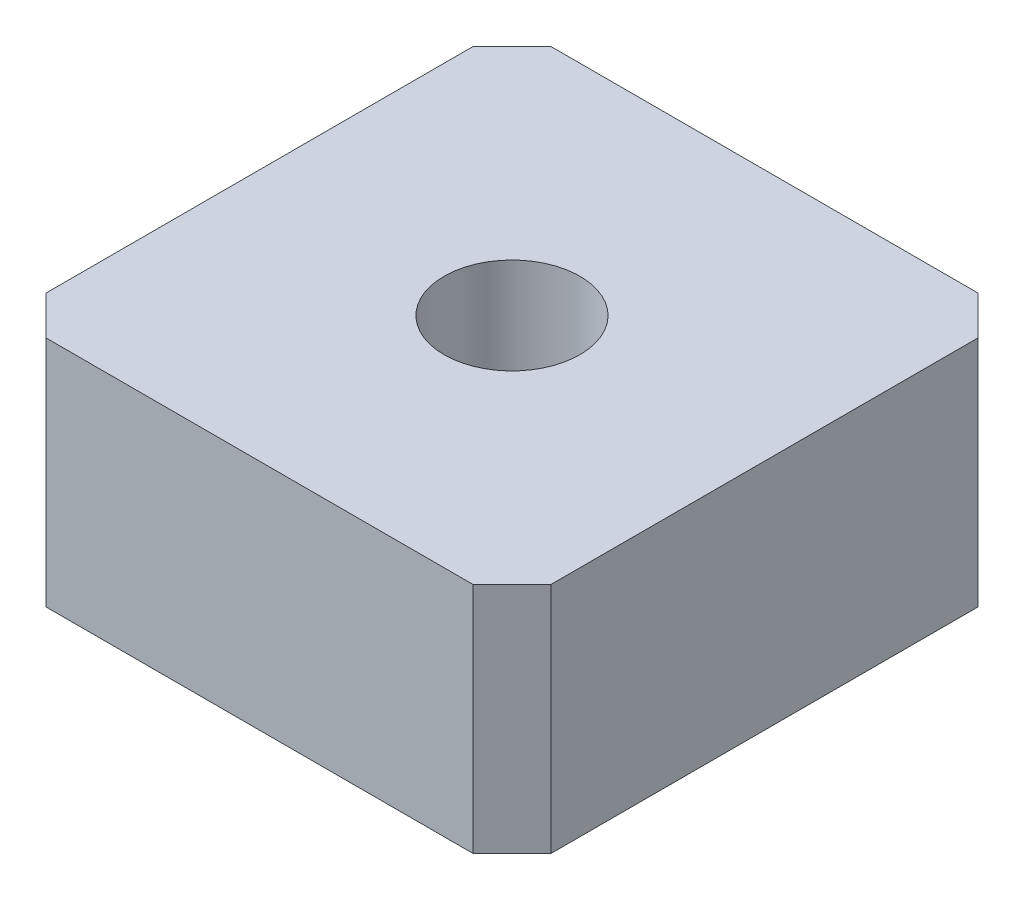
SolidWorks part; units mm, degrees
ref_plane "前视基准面" through (0, 0, 0) normal (0, 0, 1) x (1, 0, 0)
ref_plane "上视基准面" through (0, 0, 0) normal (0, 1, 0) x (1, 0, 0)
ref_plane "右视基准面" through (0, 0, 0) normal (1, 0, 0) x (0, 0, -1)
sketch "草图1" plane through (0, 0, 0) normal (0, 1, 0) x (1, 0, 0)
  line L1 (-6.5, 6.5) -> (6.5, 6.5)
  line L2 (-6.5, 6.5) -> (-6.5, -6.5)
  line L3 (-6.5, -6.5) -> (6.5, -6.5)
  line L4 (6.5, 6.5) -> (6.5, -6.5)
  line L5 (-6.5, 6.5) -> (6.5, -6.5) construction
  line L6 (-6.5, -6.5) -> (6.5, 6.5) construction
  point P0 (0, 0)
  dimension "D1" = 13
  dimension "D2" = 13
extrude "凸台-拉伸1" add sketch "草图1" along normal blind 6
hole_wizard "Ø3.5 (3.5) 直径孔1" positions "草图3" profile "草图2" hole size "Ø3.5" standard "GB" end condition through all
sketch "草图3" plane through (0, 6, 0) normal (0, 1, 0) x (1, 0, 0)
  point P0 (0, 0)
sketch "草图2" plane through (0, 6, 0) normal (1, 0, 0) x (0, 0, 1)
  line L0 (0, 0) -> (0, 6)
  line L1 (0, 6) -> (1.75, 6)
  line L2 (1.75, 6) -> (1.75, 0)
  line L5 (1.75, 0) -> (0, 0)
  line L11 (0, -6.35) -> (0, 107.95) construction
  dimension "通孔孔直径" = 3.5
  dimension "通孔孔深度" = 6
chamfer "倒角1" distance 1 angle 45 4 edges at (-6.5, 3, -6.5) (6.5, 3, -6.5) (6.5, 3, 6.5) (-6.5, 3, 6.5)
